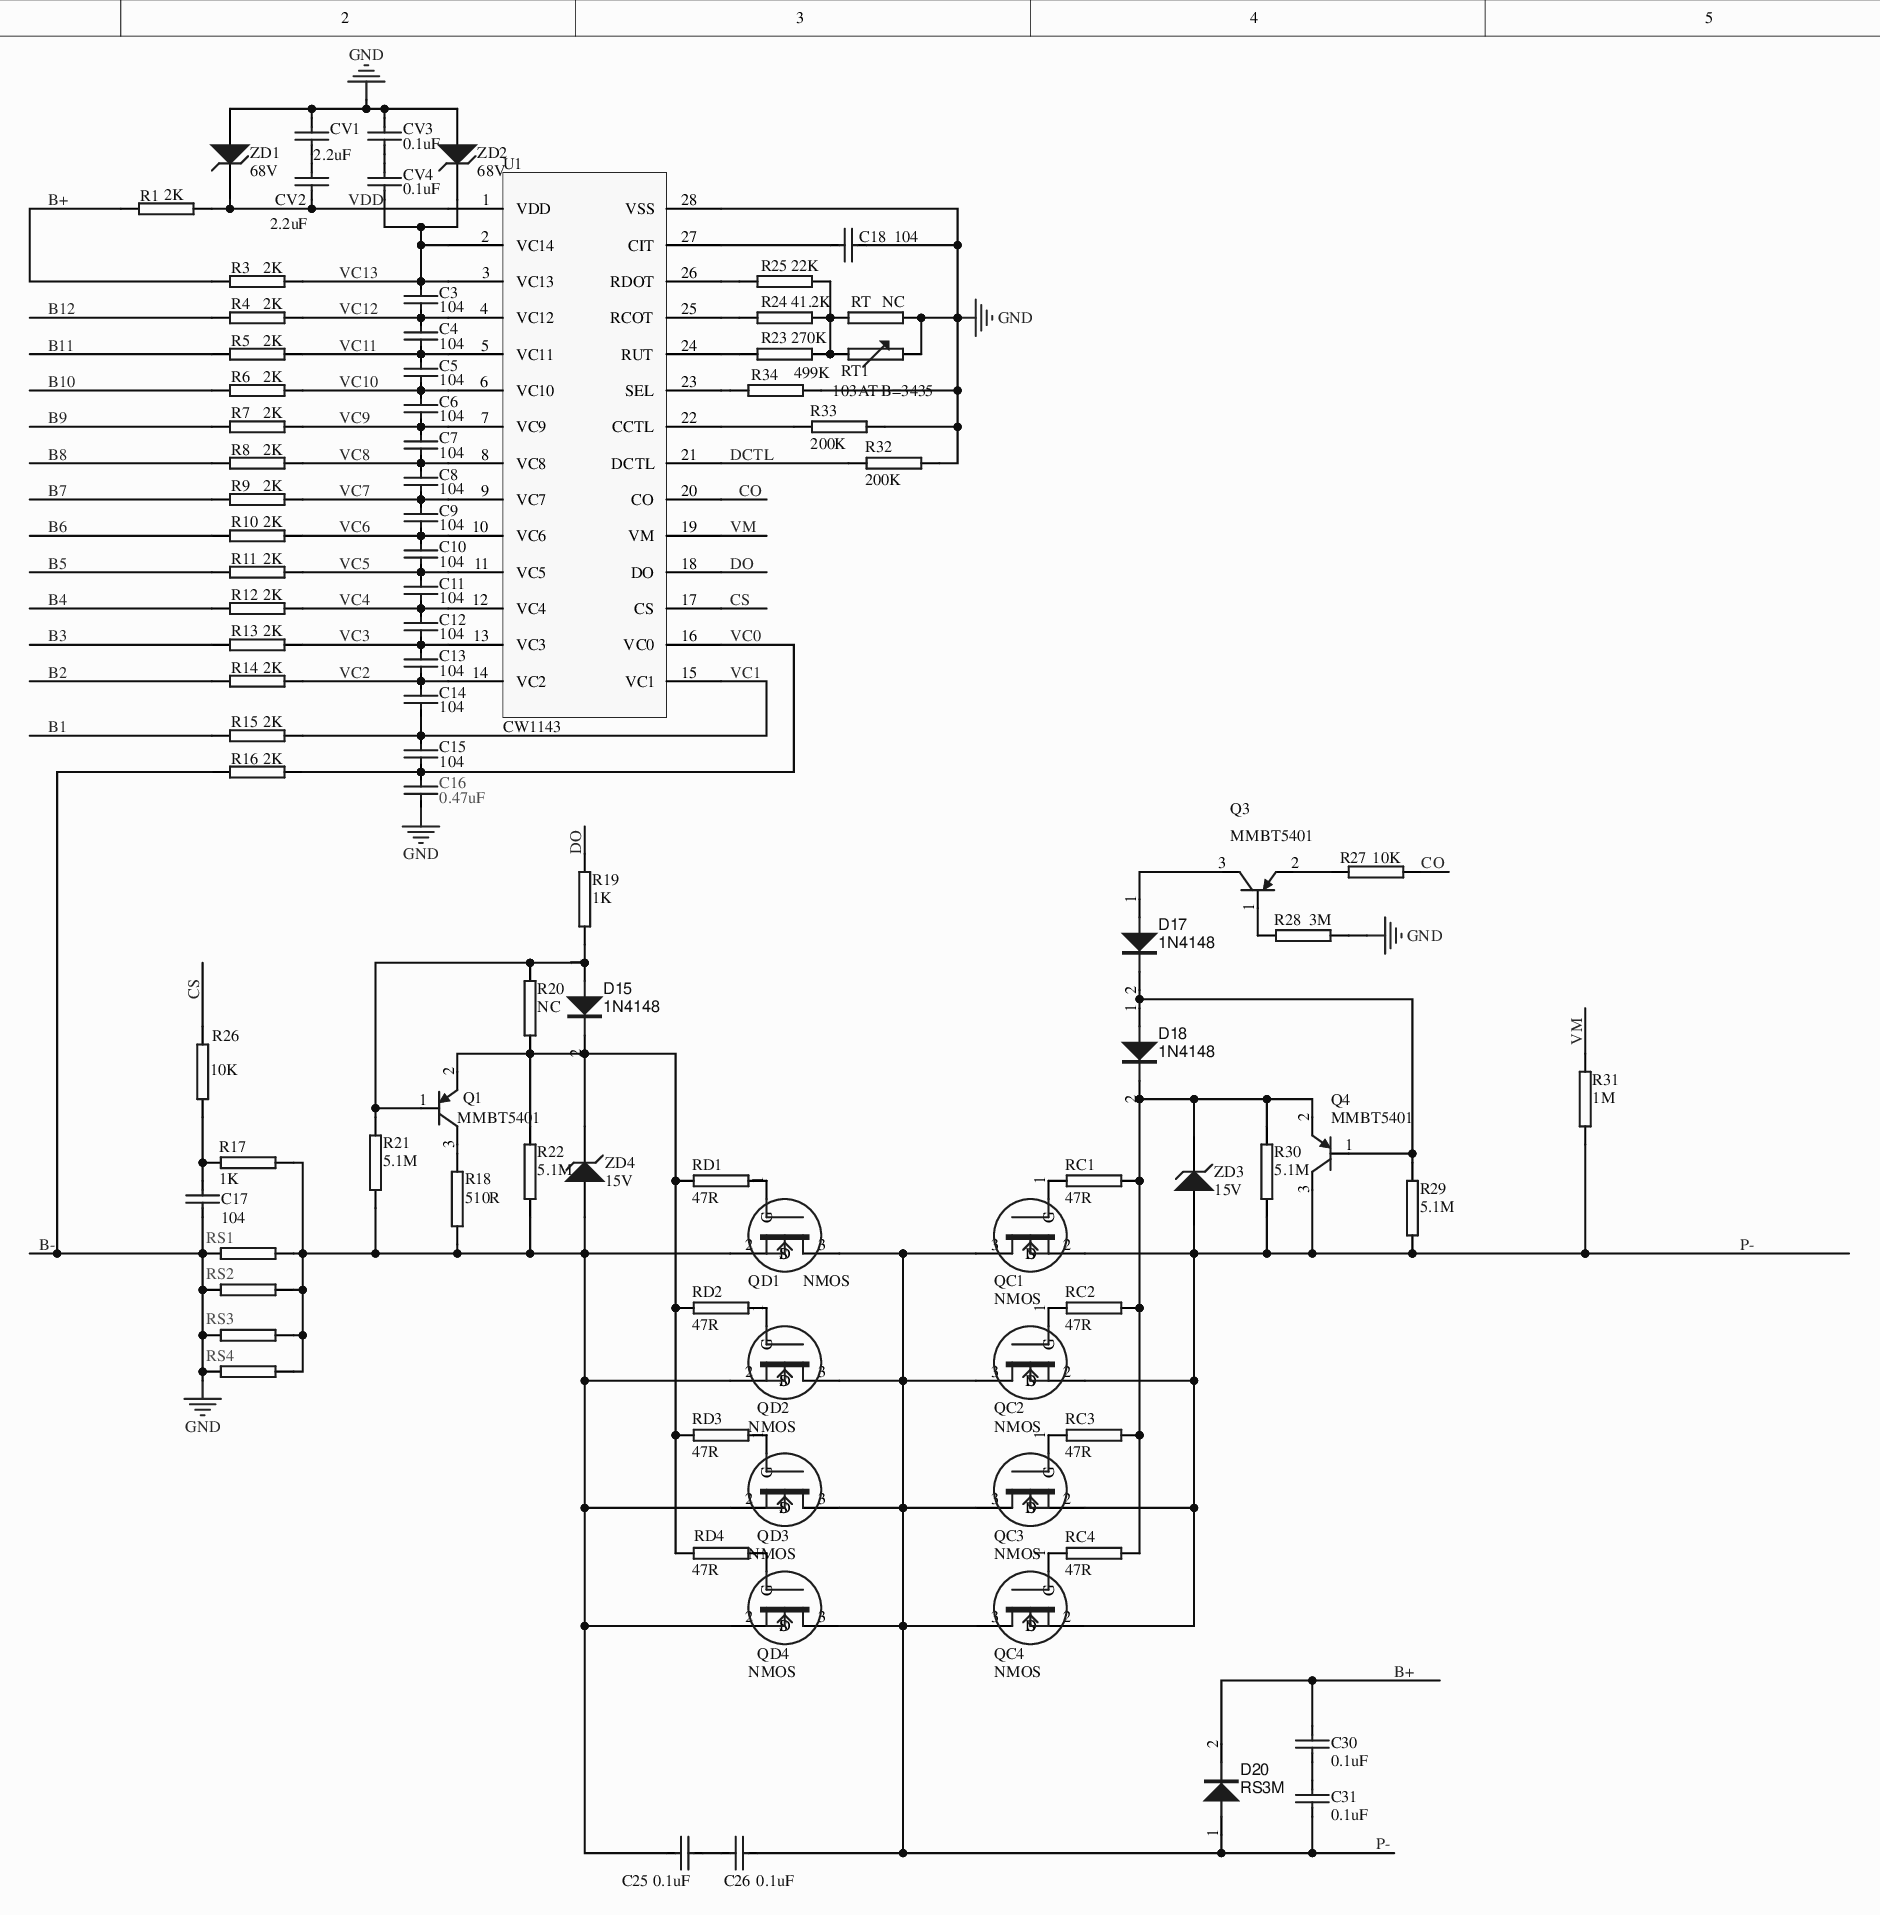
[diagram p0: MISC84391-5.SchDoc]
# Altium project MISC84391-3.PrjPcb
1 sheet, 91 parts. Net scope: global (net labels, ports and power ports of the same name join across sheets).
Board file: MISC84391.PcbDoc

## Sheet MISC84391-5.SchDoc
size 508 x 281 mm; SheetNumber: 1; SheetTotal: 1; PageSetup: Record=PageOptions¦CenterHorizontal=True¦CenterVertical=True¦PrintScale=0.77¦XCorrection=1.00¦YCorrection=1.00¦PrintKind=0¦BorderSize=5000000¦LeftOffset=0¦BottomOffset=0¦Orientation=2¦PaperLength=1000¦PaperWidth=1000¦Scale=100¦PaperSource=7¦PrintQuality=-3¦MediaType=1¦DitherType=10¦PrintScaleMode=1¦PaperKind=A4¦PaperIndex=9

### Parts
C3  104  [CAP0603]
C4  104  [CAP0603]
C5  104  [CAP0603]
C6  104  [CAP0603]
C7  104  [CAP0603]
C8  104  [CAP0603]
C9  104  [CAP0603]
C10  104  [CAP0603]
C11  104  [CAP0603]
C12  104  [CAP0603]
C13  104  [CAP0603]
C14  104  [CAP0603]
C15  104  [CAP0603]
C16  0.47uF  [CAP0603]
C17  104  [CAP0603]
C18  104  [CAP0603]
C25  0.1uF  [CAP0603]
C26  0.1uF  [CAP0603]
C30  0.1uF  [CAP0603]
C31  0.1uF  [CAP0603]
CV1  2.2uF  [CAP0805]
CV2  2.2uF  [CAP0805]
CV3  0.1uF  [CAP0603]
CV4  0.1uF  [CAP0603]
D15  1N4148  [SOD323]
D17  1N4148  [SOD323]
D18  1N4148  [SOD323]
D20  RS3M  [SMC]
Q1  MMBT5401  [SOT-23-3]
Q3  MMBT5401  [SOT-23-3]
Q4  MMBT5401  [SOT-23-3]
QC1  NMOS  [TOLL_123]
QC2  NMOS  [TOLL_123]
QC3  NMOS  [TOLL_123]
QC4  NMOS  [TOLL_123]
QD1  NMOS  [TOLL_123]
QD2  NMOS  [TOLL_123]
QD3  NMOS  [TOLL_123]
QD4  NMOS  [TOLL_123]
R1  2K  [RES0805]
R3  2K  [RES0603]
R4  2K  [RES0603]
R5  2K  [RES0603]
R6  2K  [RES0603]
R7  2K  [RES0603]
R8  2K  [RES0603]
R9  2K  [RES0603]
R10  2K  [RES0603]
R11  2K  [RES0603]
R12  2K  [RES0603]
R13  2K  [RES0603]
R14  2K  [RES0603]
R15  2K  [RES0603]
R16  2K  [RES0603]
R17  1K  [RES0603]
R18  510R  [RES0603]
R19  1K  [RES0603]
R20  NC  [RES0603]
R21  5.1M  [RES0603]
R22  5.1M  [RES0603]
R23  270K  [RES0603]
R24  41.2K  [RES0603]
R25  22K  [RES0603]
R26  10K  [RES0603]
R27  10K  [RES0603]
R28  3M  [RES0603]
R29  5.1M  [RES0603]
R30  5.1M  [RES0603]
R31  1M  [RES0603]
R32  200K  [RES0603]
R33  200K  [RES0603]
R34  499K  [RES0603]
RC1  47R  [RES0603]
RC2  47R  [RES0603]
RC3  47R  [RES0603]
RC4  47R  [RES0603]
RD1  47R  [RES0603]
RD2  47R  [RES0603]
RD3  47R  [RES0603]
RD4  47R  [RES0603]
RS1  (no value)  [2512]
RS2  (no value)  [2512]
RS3  (no value)  [2512]
RS4  (no value)  [2512]
RT  NC  [RES0603]
RT1  103AT B=3435  [WK]
U1  CW1143  [SSOP-28-0.635]
ZD1  68V  [SOD123]
ZD2  68V  [SOD123]
ZD3  15V  [SOD323]
ZD4  15V  [SOD323]

### Nets
B-: C16.2 C17.2 C18.2 CV1.1 CV3.1 R16.1 R28.1 R32.2 R33.2 R34.2 RS1.2 RS2.2 RS3.2 RS4.2 RT.2 RT1.2 U1.28(VSS) ZD1.1(A) ZD2.1(A)  [also labelled GND]
B1: R15.1
B2: R14.1
B3: R13.1
B4: R12.1
B5: R11.1
B6: R10.1
B7: R9.1
B8: R8.1
B9: R7.1
B10: R6.1
B11: R5.1
B12: R4.1
B+: C30.2 D20.2(K) R1.1 R3.1
CO: R27.2 U1.20(CO)
CS: R26.2 U1.17(CS)
DCTL: R32.1 U1.21(DCTL)
DO: R19.1 U1.18(DO)
P-: C26.2 C31.1 D20.1(A) Q4.3(C) QC1.2(S) QC1.3(D) QC2.2(S) QC2.3(D) QC3.2(S) QC3.3(D) QC4.2(S) QC4.3(D) QD1.3(D) QD2.3(D) QD3.3(D) QD4.3(D) R29.2 R30.2 R31.2 ZD3.1(A)
VC0: C15.2 C16.1 R16.2 U1.16(VC0)
VC1: C14.2 C15.1 R15.2 U1.15(VC1)
VC2: C13.2 C14.1 R14.2 U1.14(VC2)
VC3: C12.2 C13.1 R13.2 U1.13(VC3)
VC4: C11.2 C12.1 R12.2 U1.12(VC4)
VC5: C10.2 C11.1 R11.2 U1.11(VC5)
VC6: C9.2 C10.1 R10.2 U1.10(VC6)
VC7: C8.2 C9.1 R9.2 U1.9(VC7)
VC8: C7.2 C8.1 R8.2 U1.8(VC8)
VC9: C6.2 C7.1 R7.2 U1.7(VC9)
VC10: C5.2 C6.1 R6.2 U1.6(VC10)
VC11: C4.2 C5.1 R5.2 U1.5(VC11)
VC12: C3.2 C4.1 R4.2 U1.4(VC12)
VC13: C3.1 CV4.2 R3.2 U1.2(VC14) U1.3(VC13) ZD2.2(K)
VDD: CV2.2 R1.2 U1.1(VDD) ZD1.2(K)
VM: R31.1 U1.19(VM)
NetC17_1: C17.1 R17.1 R26.1
NetC18_1: C18.1 U1.27(CIT)
NetC25_1: C25.1 QD1.2(S) QD2.2(S) QD3.2(S) QD4.2(S) R17.2 R18.2 R21.2 R22.2 RS1.1 RS2.1 RS3.1 RS4.1 ZD4.1(A)
NetC25_2: C25.2 C26.1
NetC30_1: C30.1 C31.2
NetCV1_2: CV1.2 CV2.1
NetCV3_2: CV3.2 CV4.1
NetD15_1: D15.1(A) Q1.1(B) R19.2 R20.1 R21.1
NetD15_2: D15.2(K) Q1.2(E) R20.2 R22.1 RD1.1 RD2.1 RD3.1 RD4.1 ZD4.2(K)
NetD17_1: D17.1(A) Q3.3(C)
NetD17_2: D17.2(K) D18.1(A) Q4.1(B) R29.1
NetD18_2: D18.2(K) Q4.2(E) R30.1 RC1.1 RC2.1 RC3.1 RC4.1 ZD3.2(K)
NetQ1_3: Q1.3(C) R18.1
NetQ3_1: Q3.1(B) R28.2
NetQ3_2: Q3.2(E) R27.1
NetQC1_1: QC1.1(G) RC1.2
NetQC2_1: QC2.1(G) RC2.2
NetQC3_1: QC3.1(G) RC3.2
NetQC4_1: QC4.1(G) RC4.2
NetQD1_1: QD1.1(G) RD1.2
NetQD2_1: QD2.1(G) RD2.2
NetQD3_1: QD3.1(G) RD3.2
NetQD4_1: QD4.1(G) RD4.2
NetR23_1: R23.1 U1.24(RUT)
NetR23_2: R23.2 R24.2 R25.2 RT.1 RT1.1
NetR24_1: R24.1 U1.25(RCOT)
NetR25_1: R25.1 U1.26(RDOT)
NetR33_1: R33.1 U1.22(CCTL)
NetR34_1: R34.1 U1.23(SEL)

### Library data of the parts
C3-C18 C25 C26 C30 C31 CV1-CV4 = CAP
D15 D17 D18 D20 = DIODE
Q1 Q3 Q4 = PNP: PNP Bipolar Transistor; Published: 8-Jun-2000; LatestRevisionDate: 29-May-2009; LatestRevisionNote: IPC-7351 Footprint Added.; PackageVersion: Aug-1999; PackageReference: SOT-23B; PackageDescription: 3-Pin SOT-23 Package 0.95 mm Pitch, 2.4 mm Lead Span; Publisher: Altium Limited
R1 R3-R34 RC1-RC4 RD1-RD4 RS1-RS4 RT = RES
RT1 = RT1
ZD1-ZD4 = D Zener: Zener Diode; Published: 8-Jun-2000; LatestRevisionDate: 17-Jul-2002; LatestRevisionNote: Re-released for DXP Platform.; PackageReference: DIODE-0.7; PackageDescription: Diode, Thru-Hole; 2 Leads; 0.7 in Pin Spacing; Publisher: Altium Limited